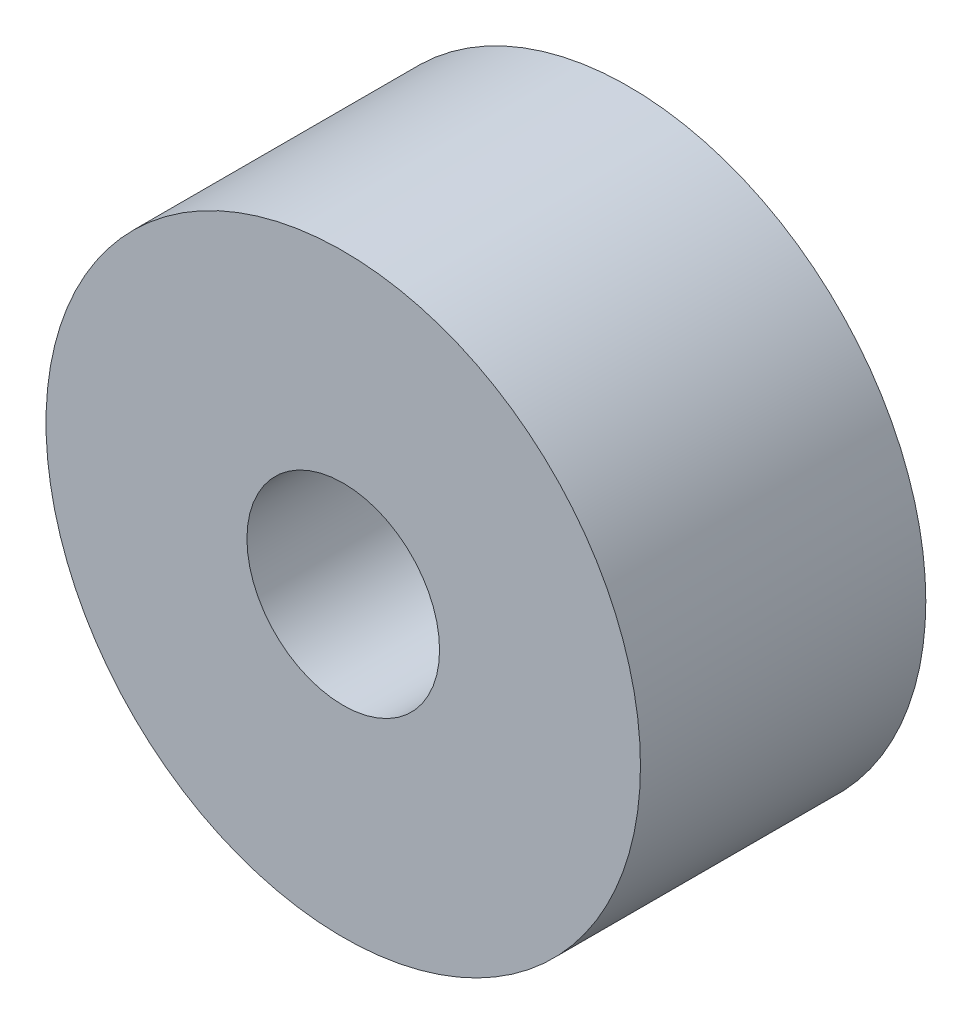
from build123d import *

# Parameters (mm, degrees)
SKETCH_1_R      = 25
SKETCH_1_R_2    = 8.1
EXTRUDE_1_DEPTH = 12


with BuildPart() as part:
    # 草图1 → 凸台-拉伸1 (new, symmetric)
    with BuildSketch(Plane.XY):
        Circle(SKETCH_1_R)
        Circle(SKETCH_1_R_2, mode=Mode.SUBTRACT)
    extrude(amount=EXTRUDE_1_DEPTH, both=True)


solid = part.part
